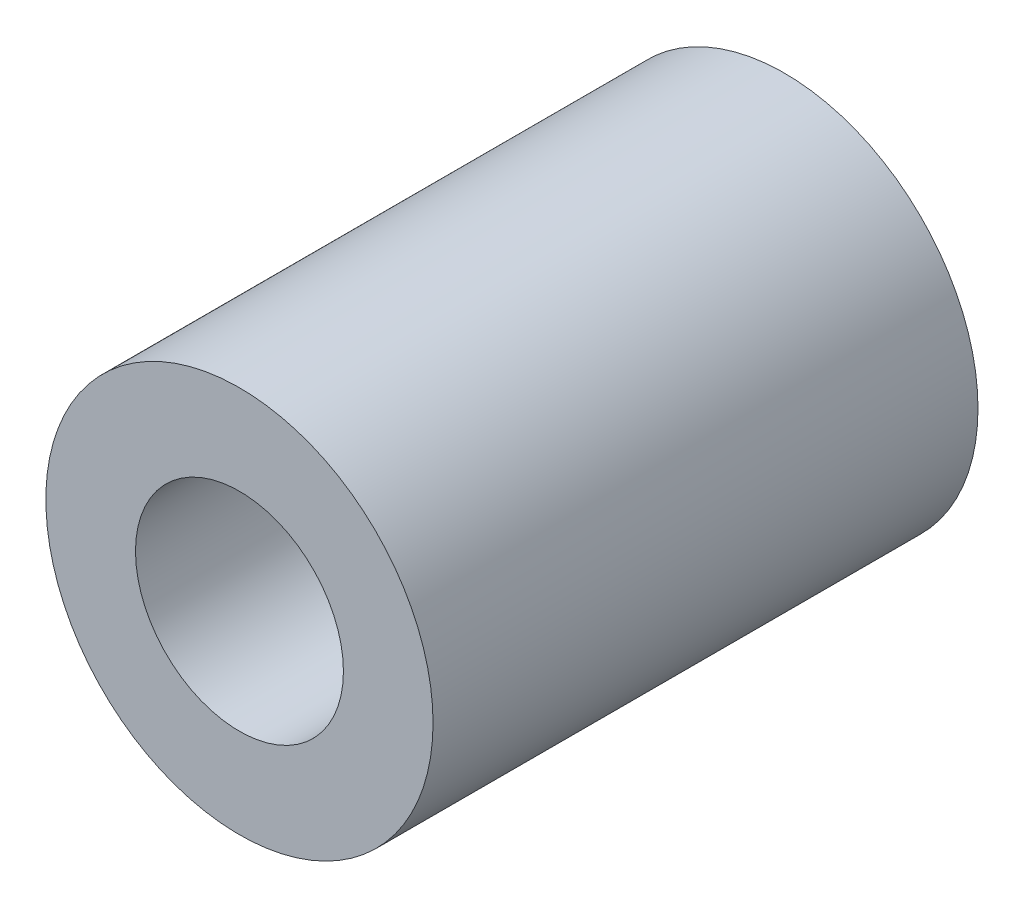
from build123d import *

# Parameters (mm, degrees)
SKETCH1_R              = 13.5
SKETCH1_R_2            = 6.5
BOSS_EXTRUDE1_DEPTH    = 38
M16X1_5_TAPPED_HOLE1_D = 14.5


with BuildPart() as part:
    # Sketch1 → Boss-Extrude1 (new body)
    with BuildSketch(Plane.XY):
        Circle(SKETCH1_R)
        Circle(SKETCH1_R_2, mode=Mode.SUBTRACT)
    extrude(amount=BOSS_EXTRUDE1_DEPTH)

    # M16x1.5 Tapped Hole1 (through all)
    with Locations(Plane(origin=(0, 0, 0), x_dir=(-1, 0, 0), z_dir=(0, 0, -1))):
        with Locations((0, 0)):
            Hole(M16X1_5_TAPPED_HOLE1_D / 2)


solid = part.part
